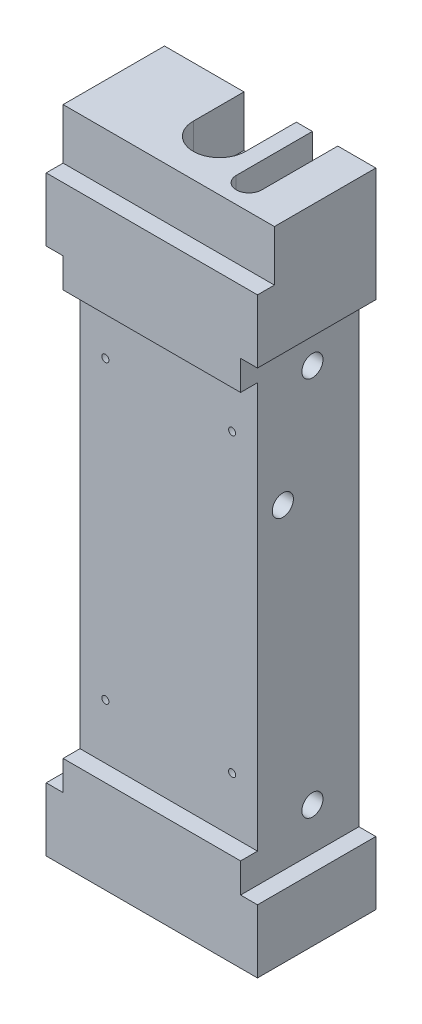
from build123d import *

# Parameters (mm, degrees)
SKETCH1_W                  = 25
SKETCH1_H                  = 12
BOSS_EXTRUDE1_DEPTH        = 77
SKETCH2_R                  = 3.1
SKETCH2_R_2                = 1.5
CUT_EXTRUDE1_DEPTH         = 79.238417673
SKETCH4_W                  = 6.2
SKETCH4_H                  = 12
SKETCH4_W_2                = 3
SKETCH4_H_2                = 18.04411339
CUT_EXTRUDE3_DEPTH         = 7
SKETCH5_W                  = 25
SKETCH5_H                  = 11
BOSS_EXTRUDE2_DEPTH        = 2
SKETCH6_W                  = 2
SKETCH6_H                  = 48
CUT_EXTRUDE4_DEPTH         = 17
M3_TAPPED_HOLE1_AT_2_COUNT = 2
M3_TAPPED_HOLE1_AT_2_PITCH = 45
M3_TAPPED_HOLE2_D          = 2.5
M3_TAPPED_HOLE2_DEPTH      = 11.5
M3_TAPPED_HOLE2_TIP        = 0.751075774
SKETCH13_W                 = 14
SKETCH13_H                 = 3.5
CUT_EXTRUDE5_DEPTH         = 2
SKETCH14_W                 = 14
SKETCH14_H                 = 3.5
CUT_EXTRUDE6_DEPTH         = 2
M3_TAPPED_HOLE3_D          = 2.5
M3_TAPPED_HOLE3_DEPTH      = 4.5
M3_TAPPED_HOLE3_TIP        = 0.751075774
SKETCH20_W                 = 25
SKETCH20_H                 = 14
CUT_EXTRUDE9_DEPTH         = 1
M3_TAPPED_HOLE5_D          = 2.5
M3_TAPPED_HOLE5_DEPTH      = 9
M3_TAPPED_HOLE5_TIP        = 0.751075774


with BuildPart() as part:
    # Sketch1 → Boss-Extrude1 (new body)
    with BuildSketch(Plane(origin=(0, 0, 0), x_dir=(1, 0, 0), z_dir=(0, 1, 0))):
        Rectangle(SKETCH1_W, SKETCH1_H)
    extrude(amount=BOSS_EXTRUDE1_DEPTH)

    # Sketch2 → Cut-Extrude1 (cut, through all)
    with BuildSketch(Plane.XZ):
        with Locations(Location((0, 0, 0), (0, 0, 270))):
            Circle(SKETCH2_R)
        with Locations(Location((6.5, 3, 0), (0, 0, 270))):
            Circle(SKETCH2_R_2)
    extrude(amount=-CUT_EXTRUDE1_DEPTH, mode=Mode.SUBTRACT)

    # Sketch4 → Cut-Extrude3 (cut)
    with BuildSketch(Plane(origin=(0, 77, 0), x_dir=(1, 0, 0), z_dir=(0, 1, 0))):
        with Locations((0, 6)):
            Rectangle(SKETCH4_W, SKETCH4_H)
        with Locations((6.5, 5.977943305)):
            Rectangle(SKETCH4_W_2, SKETCH4_H_2)
    extrude(amount=-CUT_EXTRUDE3_DEPTH, mode=Mode.SUBTRACT)

    # Sketch5 → Boss-Extrude2 (add)
    with BuildSketch(Plane.XY.offset(6)):
        with Locations((0, 5.5)):
            Rectangle(SKETCH5_W, SKETCH5_H)
        with Locations((0, 64.5)):
            Rectangle(SKETCH5_W, SKETCH5_H)
    extrude(amount=BOSS_EXTRUDE2_DEPTH)

    # Sketch6 → Cut-Extrude4 (cut)
    with BuildSketch(Plane.XY.offset(8)):
        with Locations((11.5, 35)):
            Rectangle(SKETCH6_W, SKETCH6_H)
        with Locations((-11.5, 35)):
            Rectangle(SKETCH6_W, SKETCH6_H)
    extrude(amount=-CUT_EXTRUDE4_DEPTH, mode=Mode.SUBTRACT)

    # Sketch8 → M3 Tapped Hole1 (revolve, cut)
    with BuildSketch(Plane(origin=(10.5, 57.5, -0.5), x_dir=(0, 0, -1), z_dir=(0, 1, 0))):
        Polygon((0, 0), (0, 8.251075774), (1.25, 7.5), (1.25, 0), align=None)
    m3_tapped_hole1 = revolve(axis=Axis((16.85, 57.5, -0.5), (-1, 0, 0)), mode=Mode.SUBTRACT)

    # M3 Tapped Hole1 at 2: M3 Tapped Hole1 ×2
    with Locations(*[(0, -i * M3_TAPPED_HOLE1_AT_2_PITCH, 0) for i in range(1, M3_TAPPED_HOLE1_AT_2_COUNT)]):
        add(m3_tapped_hole1, mode=Mode.SUBTRACT)

    # Mirror1: M3 Tapped Hole1 across plane
    add(m3_tapped_hole1.mirror(Plane(origin=(0, 0, 0), x_dir=(0, 0, 1), z_dir=(1, 0, 0))), mode=Mode.SUBTRACT)

    # Mirror1 copy 1 sketch → Mirror1 copy 1 (revolve, cut)
    with BuildSketch(Plane(origin=(-10.5, 12.5, -0.5), x_dir=(0, 0, -1), z_dir=(0, 1, 0))):
        Polygon((0, 0), (0, -8.251075774), (1.25, -7.5), (1.25, 0), align=None)
    revolve(axis=Axis((-16.85, 12.5, -0.5), (-1, 0, 0)), mode=Mode.SUBTRACT)

    # M3 Tapped Hole2
    with Locations(Plane(origin=(-7.5, 52.5, -6), x_dir=(-1, 0, 0), z_dir=(0, 0, -1))):
        with Locations((0, 0), (-15, 0), (-15, -35), (0, -35)):
            Hole(M3_TAPPED_HOLE2_D / 2, depth=M3_TAPPED_HOLE2_DEPTH)
            with Locations((0, 0, -(M3_TAPPED_HOLE2_DEPTH + M3_TAPPED_HOLE2_TIP / 2))):  # 118° drill point
                Cone(0, M3_TAPPED_HOLE2_D / 2, M3_TAPPED_HOLE2_TIP, mode=Mode.SUBTRACT)

    # Sketch13 → Cut-Extrude5 (cut)
    with BuildSketch(Plane(origin=(12.5, 0, 0), x_dir=(0, 0, -1), z_dir=(1, 0, 0))):
        with Locations((-1, 60.75)):
            Rectangle(SKETCH13_W, SKETCH13_H)
        with Locations((-1, 9.25)):
            Rectangle(SKETCH13_W, SKETCH13_H)
    extrude(amount=-CUT_EXTRUDE5_DEPTH, mode=Mode.SUBTRACT)

    # Sketch14 → Cut-Extrude6 (cut)
    with BuildSketch(Plane.ZY.offset(12.5)):
        with Locations((1, 60.75)):
            Rectangle(SKETCH14_W, SKETCH14_H)
        with Locations((1, 9.25)):
            Rectangle(SKETCH14_W, SKETCH14_H)
    extrude(amount=-CUT_EXTRUDE6_DEPTH, mode=Mode.SUBTRACT)

    # M3 Tapped Hole3
    with Locations(Plane(origin=(10.5, 44.955533586, 3), x_dir=(0, 1, 0), z_dir=(1, 0, 0))):
        with Locations((0, 0)):
            Hole(M3_TAPPED_HOLE3_D / 2, depth=M3_TAPPED_HOLE3_DEPTH)
            with Locations((0, 0, -(M3_TAPPED_HOLE3_DEPTH + M3_TAPPED_HOLE3_TIP / 2))):  # 118° drill point
                Cone(0, M3_TAPPED_HOLE3_D / 2, M3_TAPPED_HOLE3_TIP, mode=Mode.SUBTRACT)

    # Sketch20 → Cut-Extrude9 (cut)
    with BuildSketch(Plane(origin=(0, 77, 0), x_dir=(1, 0, 0), z_dir=(0, 1, 0))):
        with Locations((0, -1)):
            Rectangle(SKETCH20_W, SKETCH20_H)
    extrude(amount=-CUT_EXTRUDE9_DEPTH, mode=Mode.SUBTRACT)

    # M3 Tapped Hole5
    with Locations(Plane(origin=(-10.5, 35, 0), x_dir=(0, -1, 0), z_dir=(-1, 0, 0))):
        with Locations((0, 0)):
            Hole(M3_TAPPED_HOLE5_D / 2, depth=M3_TAPPED_HOLE5_DEPTH)
            with Locations((0, 0, -(M3_TAPPED_HOLE5_DEPTH + M3_TAPPED_HOLE5_TIP / 2))):  # 118° drill point
                Cone(0, M3_TAPPED_HOLE5_D / 2, M3_TAPPED_HOLE5_TIP, mode=Mode.SUBTRACT)


solid = part.part
